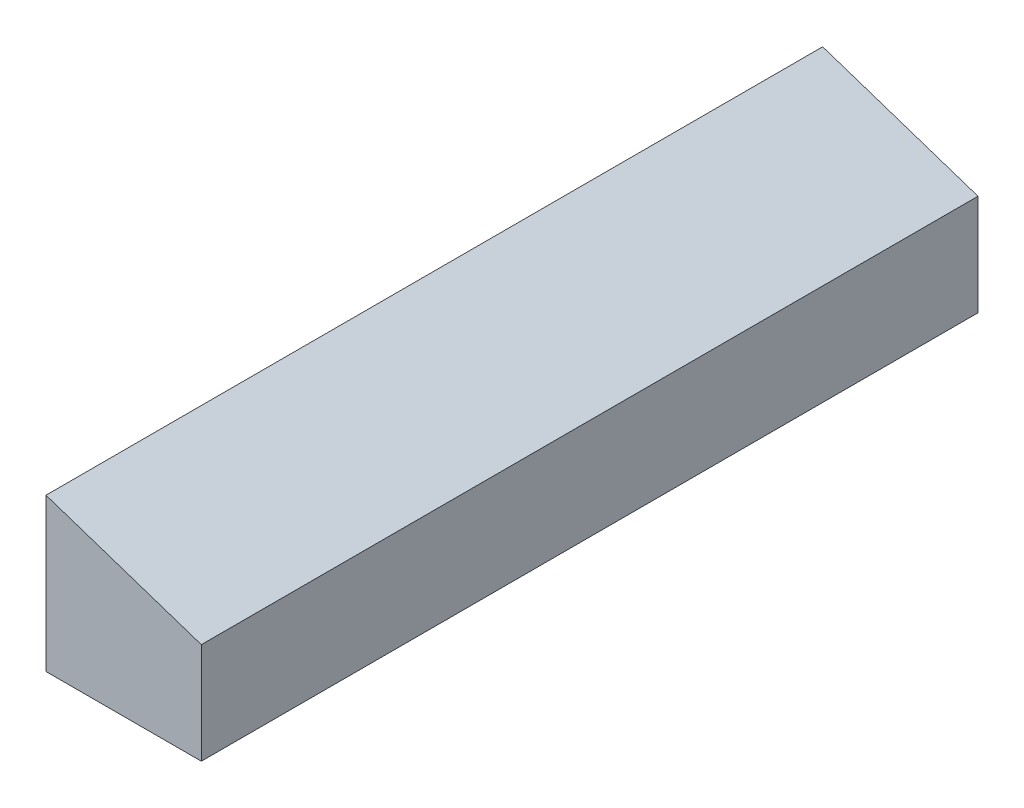
SolidWorks part; units mm, degrees
material "Q235A"
ref_plane "Front Plane" through (0, 0, 0) normal (0, 0, 1) x (1, 0, 0)
ref_plane "Top Plane" through (0, 0, 0) normal (0, 1, 0) x (1, 0, 0)
ref_plane "Right Plane" through (0, 0, 0) normal (1, 0, 0) x (0, 0, -1)
sketch "Sketch1" plane through (0, 0, 0) normal (0, 0, 1) x (1, 0, 0)
  line L0 (0, 120) -> (120, 80)
  line L1 (120, 80) -> (120, 0)
  line L2 (120, 0) -> (0, 0)
  line L3 (0, 0) -> (0, 120)
  dimension "D1" = 120
  dimension "D2" = 120
  dimension "D3" = 80
extrude "Boss-Extrude1" add sketch "Sketch1" along normal mid plane 600
shell "Shell1" thickness 2
sketch "Sketch2" plane through (0, 0, 0) normal (0, -1, 0) x (1, 0, 0)
  line L1 (120, 300) -> (0, 300)
  line L2 (120, 300) -> (120, -300)
  line L3 (120, -300) -> (0, -300)
  line L4 (0, 300) -> (0, -300)
extrude "Cut-Extrude1" cut sketch "Sketch2" against normal up to surface (2 mm away) up to face at (59, 2, 0)
